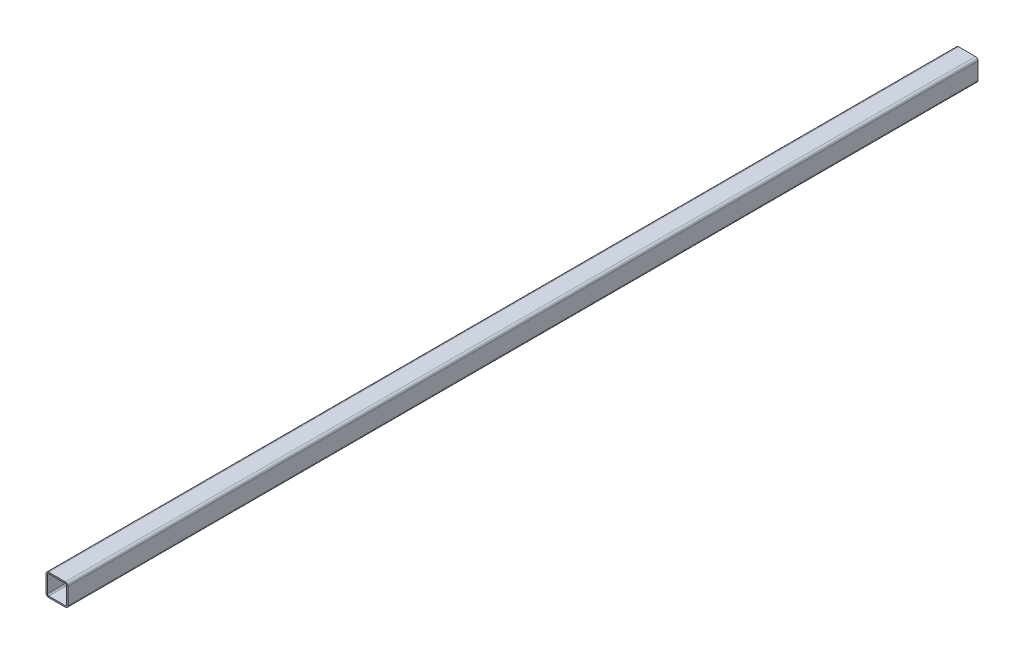
from build123d import *

# Parameters (mm, degrees)
GB_6728_1986_050_X_50_X_3_1_DEPTH = 2070


with BuildPart() as part:
    # Sketch1 → Gb／6728-1986方形空心型钢 050 X 50 X 3(1) (new body)
    with BuildSketch(Plane.YX.offset(-1035)):
        with BuildLine():
            Line((-19, -25), (19, -25))
            ThreePointArc((19, -25), (23.242640687, -23.242640687), (25, -19))
            Line((25, -19), (25, 19))
            ThreePointArc((25, 19), (23.242640687, 23.242640687), (19, 25))
            Line((19, 25), (-19, 25))
            ThreePointArc((-19, 25), (-23.242640687, 23.242640687), (-25, 19))
            Line((-25, 19), (-25, -19))
            ThreePointArc((-25, -19), (-23.242640687, -23.242640687), (-19, -25))
        make_face()
        with BuildLine():
            Line((-19, -22), (19, -22))
            ThreePointArc((19, -22), (21.121320344, -21.121320344), (22, -19))
            Line((22, -19), (22, 19))
            ThreePointArc((22, 19), (21.121320344, 21.121320344), (19, 22))
            Line((19, 22), (-19, 22))
            ThreePointArc((-19, 22), (-21.121320344, 21.121320344), (-22, 19))
            Line((-22, 19), (-22, -19))
            ThreePointArc((-22, -19), (-21.121320344, -21.121320344), (-19, -22))
        make_face(mode=Mode.SUBTRACT)
    extrude(amount=GB_6728_1986_050_X_50_X_3_1_DEPTH)


solid = part.part
